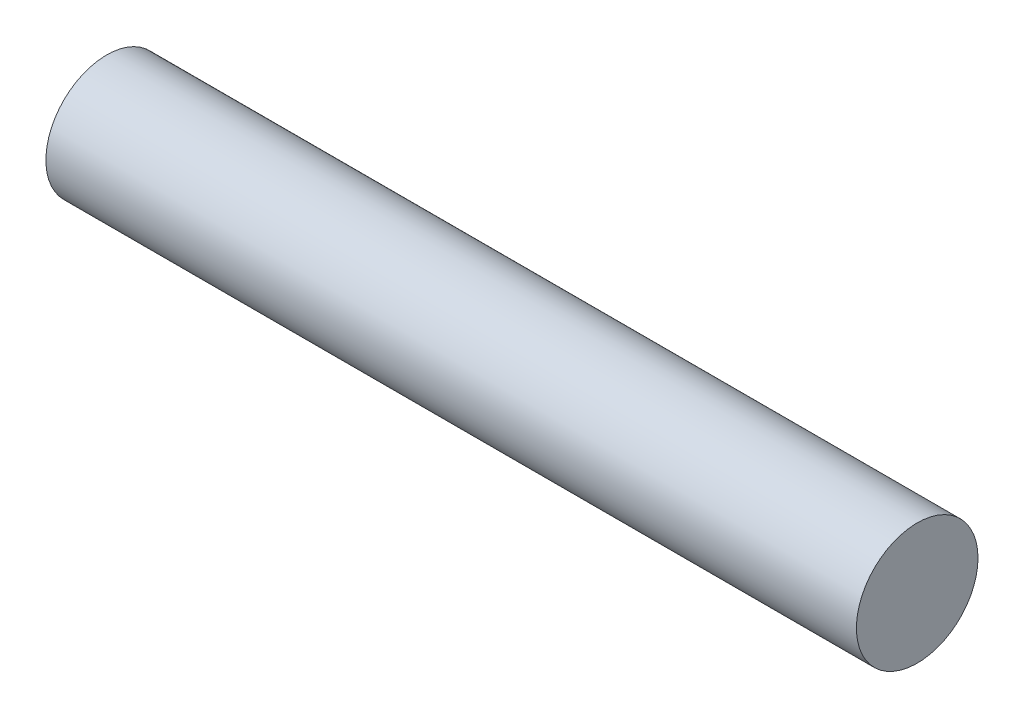
SolidWorks part; units mm, degrees
ref_plane "Front Plane" through (0, 0, 0) normal (0, 0, 1) x (1, 0, 0)
ref_plane "Top Plane" through (0, 0, 0) normal (0, 1, 0) x (1, 0, 0)
ref_plane "Right Plane" through (0, 0, 0) normal (1, 0, 0) x (0, 0, -1)
sketch "Sketch1" plane through (0, 0, 0) normal (1, 0, 0) x (0, 0, -1)
  circle A0 centre (0, 0) radius 1.5
  dimension "D1" = 3
extrude "Boss-Extrude1" add sketch "Sketch1" along normal blind 20
